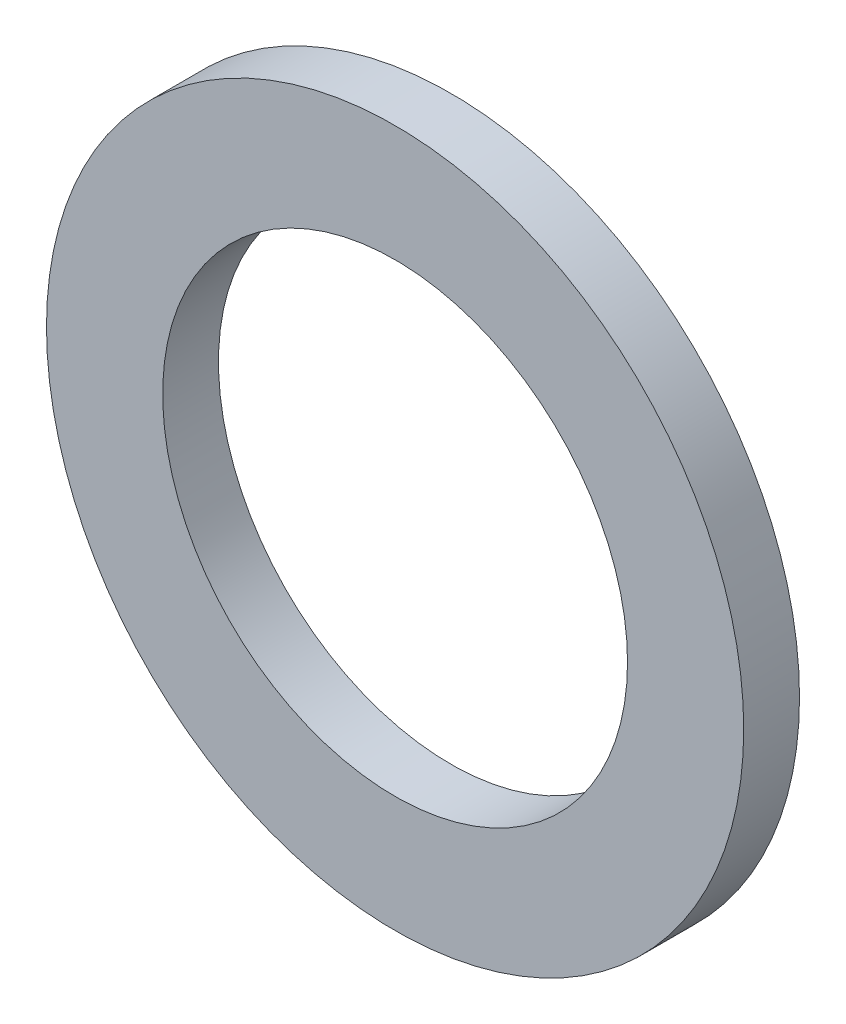
from build123d import *

# Parameters (mm, degrees)
SKETCH1_R           = 75
SKETCH1_R_2         = 50
BOSS_EXTRUDE1_DEPTH = 12


with BuildPart() as part:
    # Sketch1 → Boss-Extrude1 (new body)
    with BuildSketch(Plane.XY):
        Circle(SKETCH1_R)
        Circle(SKETCH1_R_2, mode=Mode.SUBTRACT)
    extrude(amount=BOSS_EXTRUDE1_DEPTH)


solid = part.part
